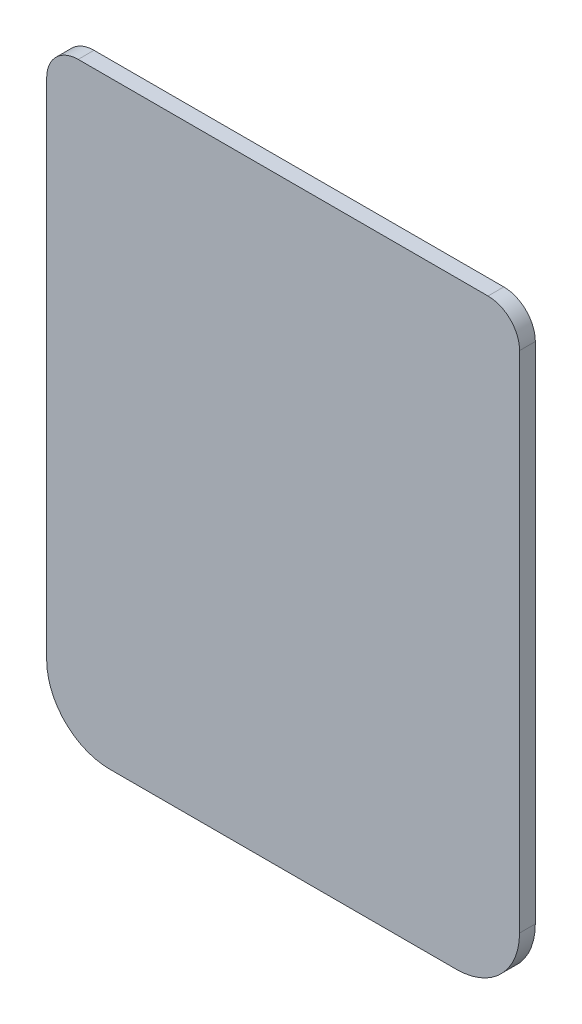
from build123d import *

# Parameters (mm, degrees)
SKETCH1_W           = 150
SKETCH1_H           = 190
BOSS_EXTRUDE1_DEPTH = 5
FILLET1_R           = 10
FILLET2_R           = 20


with BuildPart() as part:
    # Sketch1 → Boss-Extrude1 (new body)
    with BuildSketch(Plane.XY):
        Rectangle(SKETCH1_W, SKETCH1_H)
    extrude(amount=BOSS_EXTRUDE1_DEPTH)

    # Fillet1
    fillet1_edges = [part.edges().sort_by_distance(p)[0] for p in [
        (-75, 95, 2.5),
        (75, 95, 2.5),
    ]]
    fillet(fillet1_edges, radius=FILLET1_R)

    # Fillet2
    fillet2_edges = [part.edges().sort_by_distance(p)[0] for p in [
        (75, -95, 2.5),
        (-75, -95, 2.5),
    ]]
    fillet(fillet2_edges, radius=FILLET2_R)


solid = part.part
